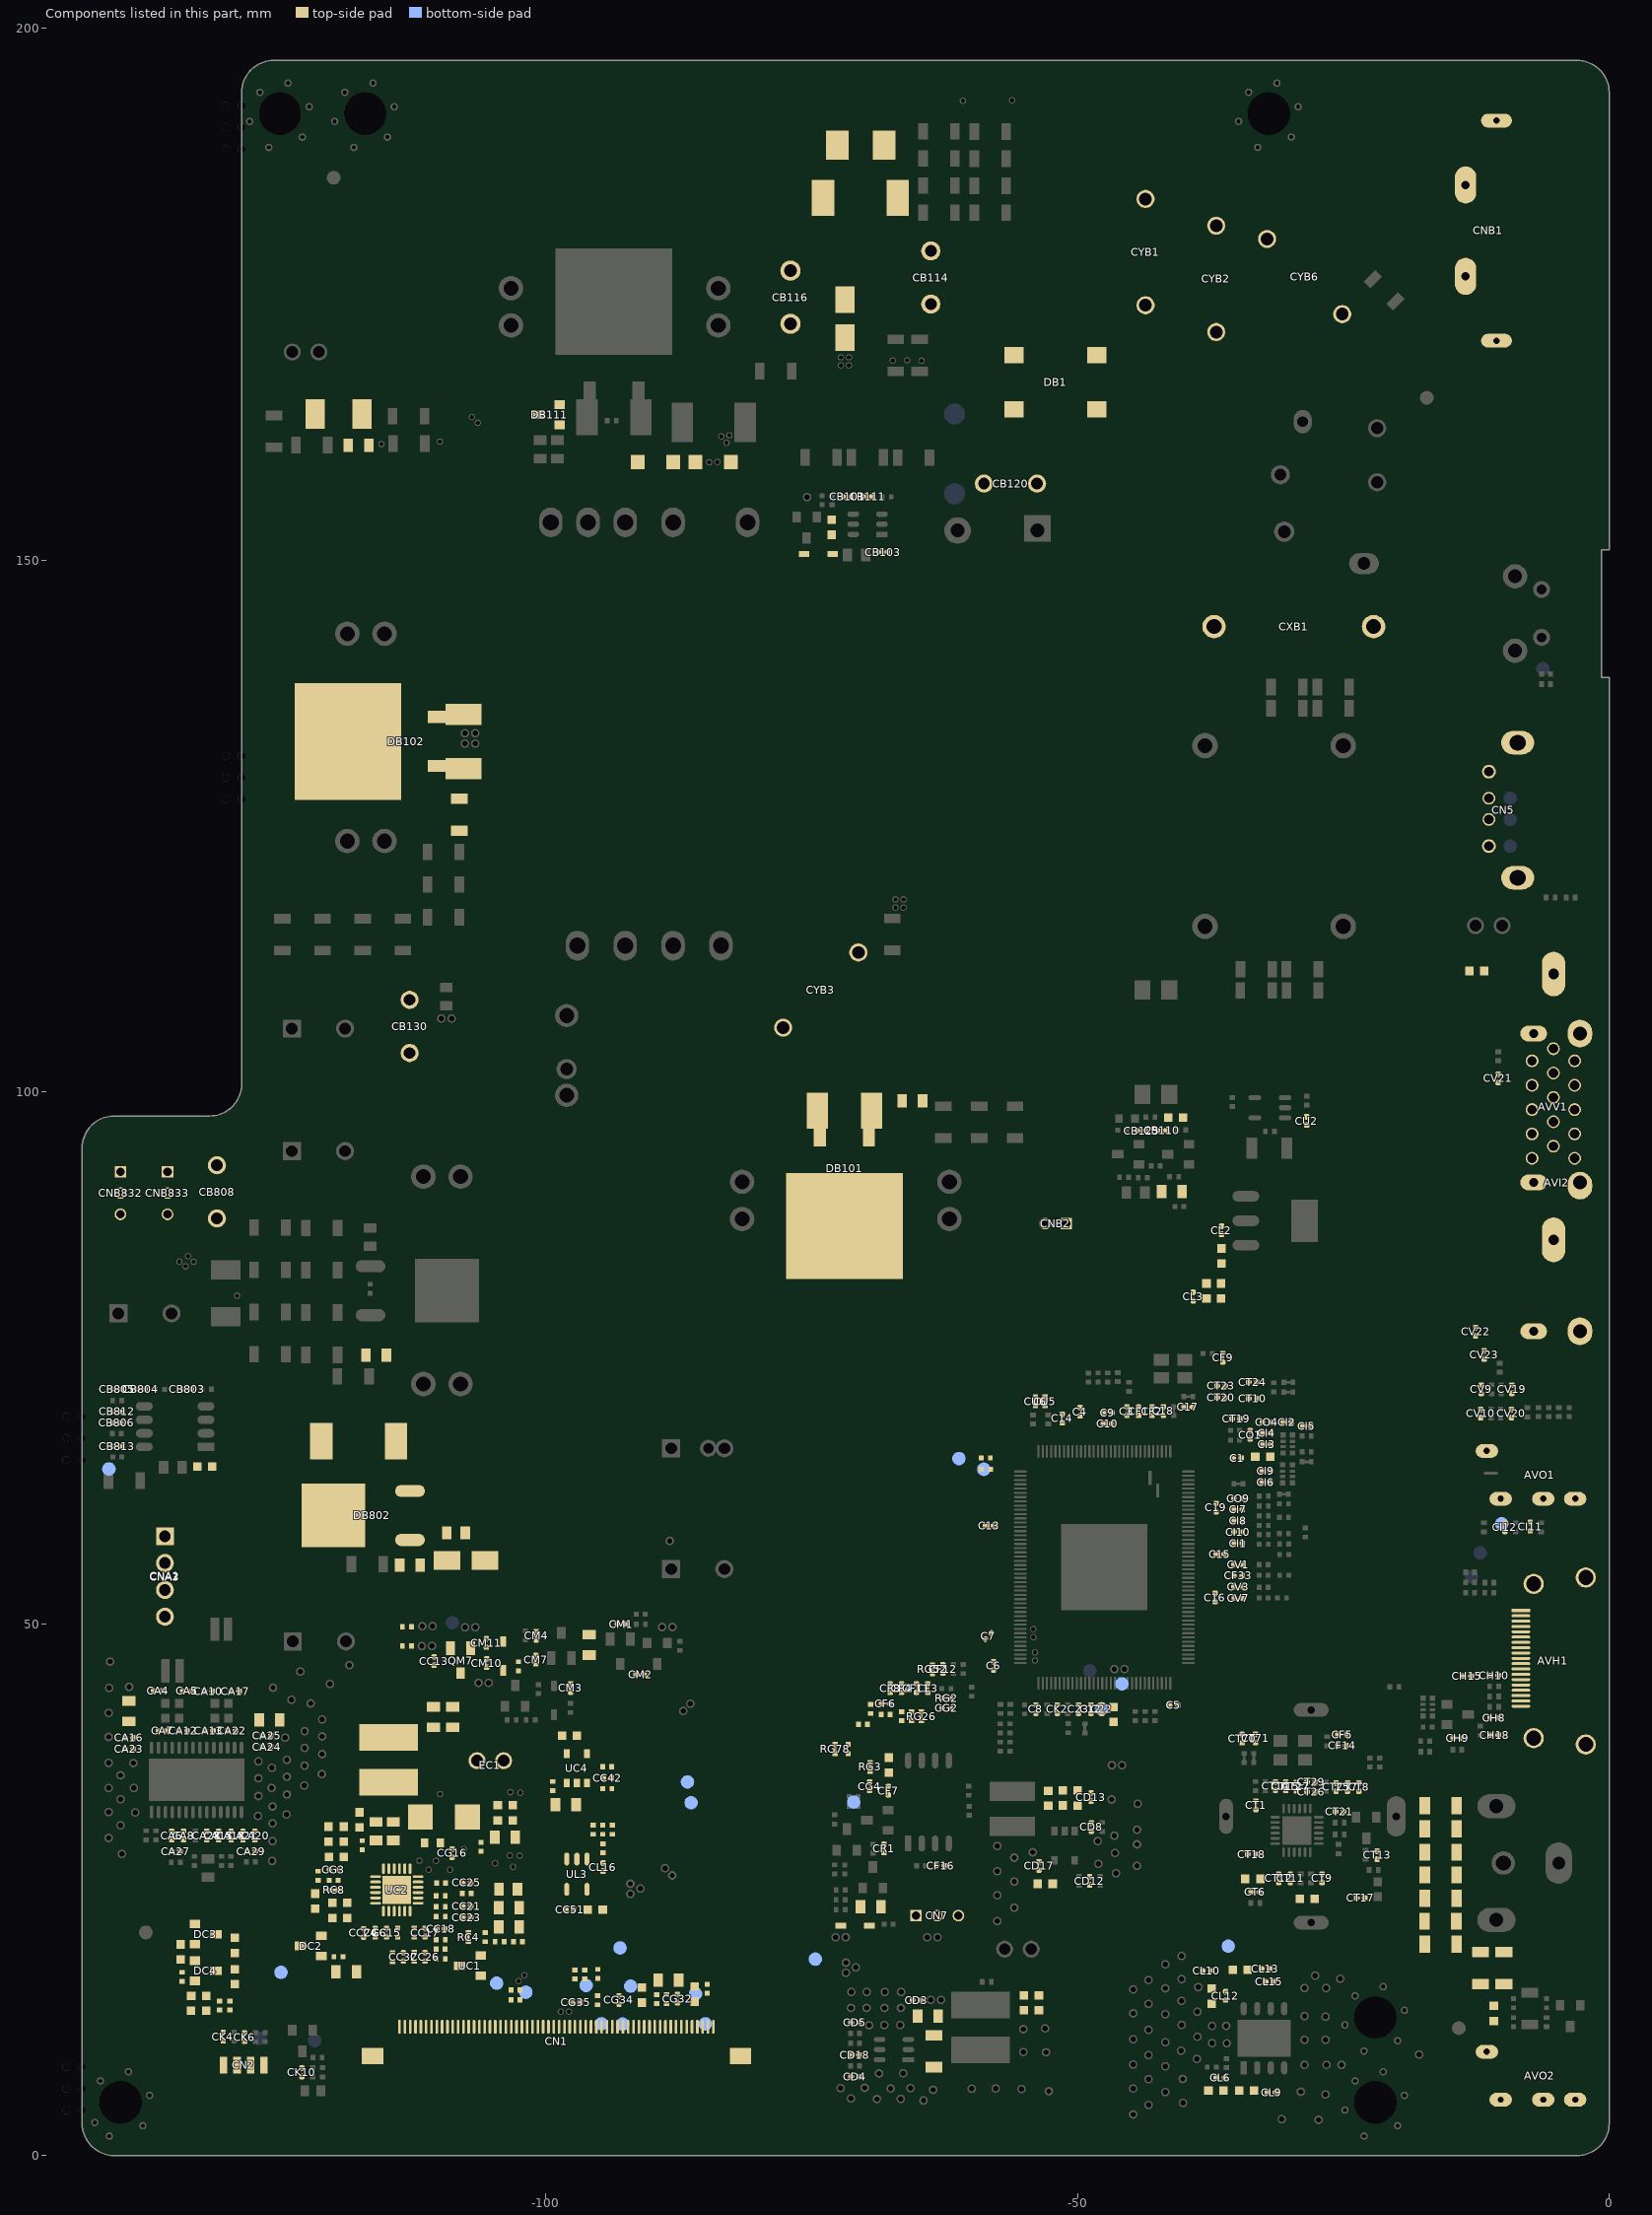
[diagram p0: the components of this part, seen from the top]
# Altium PCB MISC86383-9.PcbDoc (part 2 of 18)
Units mm, origin at the board's own origin, x right, y up, seen from the top; angles counter-clockwise.
Board outline 143.6 x 197 mm, 2 copper layers (TopLayer, BottomLayer), stack 1.571 mm thick; 743 components, 401 nets, 2996 pads, 1077 vias.
Unrouted connection lines stored in the file: 4.

## Classes and differential pairs (continued)
component class TV#08_TCON: AVDD CC1 CC2 CC4 CC5 CC7 CC8 CC9 CC10 CC11 CC12 CC13 CC15 CC17 CC18 CC19 CC20 CC21 CC23 CC24 CC25 CC26 CC27 CC29 CC30 CC31 CC32 CC33 CC34 CC38 CC42 CC43 CC50 CC51 CG3 CG4 CG6 CG14 CG16 CG22 CG28 CG31 CG32 CG33 CG34 CG35 CL16 CM10 CM11 CN1 CPV CPV2 DC1 DC2 DC3 DC4 DM3 DVDD EC1 GREF LC1 OE1 POL QM7 RC1 RC2 RC3 RC4 RC8 RC10 RC12 RC13 RC14 RC15 RC18 RC19 RC20 RC23 RC24 RC27 RC31 RC32 RC33 RC35 RC36 RG2 RG3 RG5 RG6 RG7 RG8 RG9 RG12 RG13 RG14 RG15 RG16 RG21 RG22 RG25 RG26 RG39 RG40 RG41 RG42 RG43 RG44 RG46 RG48 RG49 RG52 RG58 RG59 RG60 RG61 RG62 RG63 RG78 RG82 RGV1 RL3 RL7 RL50 RL51 RM12 STV TP TVCOM UC1 UC2 UC4 UL3 VMID/SCL VMID/SDA VOFF VON XAO
component class TV#09_LevelShif_DS8926B: RG82 STV
component class TV#10_FFC_LRbord: CNL2 CNL3
component class PS#01_XXXXXXXXXXXXXXX: "Conformal Coating" CYB5 EB107 EB801+ EB801- EVA3 EVA4 EVA5 EVA6 GL7 ML1 RB111 RB113 ZDB2
net class HOT: 12V-OVP BRO D_QB101 L L-1 L-2 L-N N N-1 N-2 N-3 NetBB101_2 NetCB101_1 NetCB103_1 NetCB113_1 NetCB113_2 NetCB114_1 NetCB114_2 NetCB116_1 NetCB116_2 NetCYB3_1 NetDB104_K NetDB106_K NetDB109_A NetDB109_K NetDB111_1 NetDB111_2 NetDB112_K NetRB101_2 NetRB106_1 NetRB141_1 NetRB143_1 NetRB144_1 NetRB150_1 SGND VBRIDGE VCC
net class POWER: 12V 12V-OVP BRO D_QB101 D_QB801 GND GND1 L L-1 L-2 L-N LED+ LED_CS LED_FB LED_GATE LED_OVP N N-1 N-2 N-3 NetBB101_2 NetBB801_2 NetBB803_1 NetCB101_1 NetCB103_1 NetCB109_1 NetCB109_2 NetCB113_1 NetCB113_2 NetCB114_1 NetCB114_2 NetCB115_1 NetCB116_1 NetCB116_2 NetCB117_1 NetCB117_2 NetCB118_1 NetCB118_2 NetCB125_1 NetCB125_2 NetCB801_2 NetCB803_1 NetCB804_1 NetCB805_2 NetCB809_1 NetCB810_2 NetCB812_2 NetCB813_2 NetCNB1_3 NetCNB1_4 NetCYB3_1 NetDB104_K NetDB106_K NetDB109_A NetDB109_K NetDB111_1 NetDB111_2 NetDB112_K NetQB105_C NetQB801_G NetRB101_2 NetRB106_1 NetRB141_1 NetRB143_1 NetRB144_1 NetRB150_1 PS_ON PWM_REF SGND STY VBL VBRIDGE VCC

## Components (designator, comment, footprint, x,y, rotation, side; value= is the part's Value field where it differs from the comment)
1.15V_STB "TEST" TP -45.822,44.348 r90 bottom
3V3_STB "TEST" TP -47.752,42.012 r180 bottom
3V3_TUNER "TEST" TP -35.82,19.686 r90 bottom
5V_STB "TEST" TP -74.651,18.466 r90 bottom
AI_V "AI_GRIPPER_V" AI_GRIPPER_V 483.311,-17.234 r270 top
AVDD "TEST" TP -101.879,15.354 r180 bottom
AVH1 "HDMI jack,HDMI Jack,H,Block up,SMD,51U019S-313HFN-E-R-F,FREEPORT" HDMI-HS-11 -0.6,46.5 r90 top locked
AVI2 "RCA jack,RCA Jack,AV3,H,Red、White、Yellow,CH5.5,D14,Seal,DIP,AV3-8.4-15C red/white/yellow,JSL" AV3-H14-15 0,91.5 r90 top locked
AVO1 "Earphone jack,Earphone Jack,H,Φ3.6,CH5.5,Black,Seal,DIP,PJ-320B-Φ5.5,JSL" PHONE-HD-43 0,64 r90 top locked
AVO2 "NC/Earphone jack,Earphone Jack,H,Φ3.6,CH5.5,Black,Seal,DIP,PJ-320B-Φ5.5,JSL" PHONE-HD-43 0,7.5 r90 top locked
AVV1 "NC/WLHD-051A" DB15-HF-1 0,98.6 r90 top locked
BB101 "Ferrite bead,BEAD,50ohm,3.0×4.0mm,9A,SMD,TP,BPH403025W4-470T,TAI-TECH" L(4*3*2.55)-S -71.882,172.733 r270 top
BB801 "Ferrite bead,BEAD,80ohm,0805,4000mA,SMD,TP,UPZ2012D800-4R0TF,Sunlord" R0805 -108.445,58.534 r180 top
BB802 "NC/Ferrite bead,BEAD,50ohm,3.0×4.0mm,9A,SMD,TP,BPH403025W4-470T,TAI-TECH" L(4*3*2.55)-S -107.505,55.956 r180 top
C1 "1uF-0402-X5R-±20%-6.3V" C0402 -34.985,65.586 r180 top
C2 "NC/10uF-0603-X5R-±20%-6.3V" C0603 -32.571,65.699 r0 top
C3 "1uF-0402-X5R-±20%-6.3V" C0402 -45.337,69.994 r270 top
C4 "1uF-0402-X5R-±20%-6.3V" C0402 -49.757,69.931 r270 top
C5 "1uF-0402-X5R-±20%-6.3V" C0402 -40.956,42.333 r180 top
C6 "Ceramic capacitor,CAP MC,16V,0.1uF,±10%,X7R,0402,SMD,TP" C0402 -57.891,46.047 r90 top
C7 "Ceramic capacitor,CAP MC,16V,0.1uF,±10%,X7R,0402,SMD,TP" C0402 -58.38,48.848 r45 top
C8 "Ceramic capacitor,CAP MC,16V,0.1uF,±10%,X7R,0402,SMD,TP" C0402 -53.91,41.978 r90 top
C9 "1uF-0402-X5R-±20%-6.3V" C0402 -47.159,69.844 r0 top
C10 "1uF-0402-X5R-±20%-6.3V" C0402 -47.165,68.815 r0 top
C11 "10uF-0603-X5R-±20%-6.3V" C0603 -46.607,41.47 r90 top
C12 "1uF-0402-X5R-±20%-6.3V" C0402 -48.728,41.978 r90 top
C13 "Ceramic capacitor,CAP MC,16V,0.1uF,±10%,X7R,0402,SMD,TP" C0402 -58.278,59.212 r0 top
C14 "Ceramic capacitor,CAP MC,16V,0.1uF,±10%,X7R,0402,SMD,TP" C0402 -51.435,69.31 r270 top
C15 "Ceramic capacitor,CAP MC,16V,0.1uF,±10%,X7R,0402,SMD,TP" C0402 -36.576,56.54 r180 top
C16 "Ceramic capacitor,CAP MC,16V,0.1uF,±10%,X7R,0402,SMD,TP" C0402 -37.059,52.476 r270 top
C17 "Ceramic capacitor,CAP MC,16V,0.1uF,±10%,X7R,0402,SMD,TP" C0402 -39.586,70.371 r0 top
C18 "Ceramic capacitor,CAP MC,16V,0.1uF,±10%,X7R,0402,SMD,TP" C0402 -41.912,70.002 r270 top
C19 "Ceramic capacitor,CAP MC,16V,0.1uF,±10%,X7R,0402,SMD,TP" C0402 -36.944,60.935 r90 top
C22 "NC/1uF-0402-X5R-±20%-6.3V" C0402 -47.725,41.978 r90 top
C23 "Ceramic capacitor,CAP MC,16V,0.1uF,±10%,X7R,0402,SMD,TP" C0402 -49.909,41.978 r90 top
CA4 "2200pF-0402-X7R-±10%-50V" C0402 -136.495,43.698 r180 top
CA5 "2200pF-0402-X7R-±10%-50V" C0402 -133.739,43.673 r0 top
CA6 "0.22uF-0402-X5R-±10%-16V" C0402 -135.182,30.084 r270 top
CA7 "0.22uF-0402-X5R-±10%-16V" C0402 -136.045,39.939 r0 top
CA8 "0.22uF-0402-X5R-±10%-16V" C0402 -134.064,30.084 r270 top
CA10 "2200pF-0402-X7R-±10%-50V" C0402 -131.732,43.66 r180 top
CA12 "0.22uF-0402-X5R-±10%-16V" C0402 -134.115,39.939 r180 top
CA13 "0.22uF-0402-X5R-±10%-16V" C0402 -131.677,39.939 r0 top
CA15 "Ceramic capacitor,CAP MC,16V,0.1uF,±10%,X7R,0402,SMD,TP" C0402 -130.762,30.084 r270 top
CA16 "NC/1000pF-0402-X7R-±10%-50V" C0402 -139.191,39.278 r0 top
CA17 "2200pF-0402-X7R-±10%-50V" C0402 -129.205,43.66 r180 top
CA18 "NC/1uF-0402-X5R-±20%-16V" C0402 -129.594,30.084 r270 top
CA20 "0.22uF-0402-X5R-±10%-16V" C0402 -127.359,30.084 r270 top
CA21 "0.22uF-0402-X5R-±10%-16V" C0402 -128.476,30.084 r270 top
CA22 "0.22uF-0402-X5R-±10%-16V" C0402 -129.543,39.939 r180 top
CA23 "NC/0.1uF-0402-X5R-±20%-16V" C0402 -139.191,38.212 r0 top
CA24 "Ceramic capacitor,CAP MC,16V,0.1uF,±10%,X7R,0402,SMD,TP" C0402 -126.233,38.427 r180 top
CA25 "NC/1000pF-0402-X7R-±10%-50V" C0402 -126.233,39.494 r180 top
CA27 "3300pF-0402-X7R-±10%-50V" C0402 -134.782,28.598 r0 top
CA28 "1uF-0402-X5R-±20%-16V" C0402 -131.88,30.084 r90 top
CA29 "3300pF-0402-X7R-±10%-50V" C0402 -127.71,28.604 r180 top
CA31 "10uF-0805-X5R-±20%-16V" C0805 -139.212,41.78 r270 top
CA32 "NC/10uF-0805-X5R-±20%-16V" C0805 -125.979,40.955 r180 top
CA36 "NC/10uF-0805-X5R-±20%-16V" C0805 -69.448,23.398 r0 top
CAUTION "CAUTION" CAUTION -173.126,207.416 r180 bottom
CB101 "100pF-0402-NPO-±5%-50V" C0402 -71.641,155.994 r0 top
CB102 "0.1uF-0603-X7R-±10%-50V" C0603 -73.114,153.111 r90 top
CB103 "Ceramic capacitor,CAP MC,50V,1000pF,±10%,X7R,0402,SMD,TP" C0402 -68.288,150.774 r180 top
CB109 "Ceramic capacitor,CAP MC,25V,0.22uF,±10%,X7R,0603,SMD,TP" C0603 -40.767,97.612 r0 top
CB110 "NC/1000pF-0402-X7R-±10%-50V" C0402 -42.062,96.393 r0 top
CB111 "NC/Ceramic capacitor,CAP MC,50V,100pF,±5%,NPO,0402,SMD,TP" C0402 -69.736,155.994 r180 top
CB113 "NC/220PF-0805-NPO-±10%-200V" C0805 -117.615,160.807 r180 top
CB114 "Film capacitor,CAP PE,400V,4700pF,±5%,P,5.0mm,PC,DIP,TP,Fara" CAP8*2.5-V-5 -63.792,176.593 r90 top
CB115 "0.1uF-0805-X7R-±10%-50V" C0805 -41.123,90.627 r180 top
CB116 "Ceramic capacitor,CAP CD,2KV,68pF,±5%,SL,IK,5.0mm,DIP,TP,Walsin" CAP6.5*5-V-5-1 -76.987,174.739 r90 top
CB117 "1000pF-0805-NPO-±10%-200V" C0805 -65.532,99.187 r0 top
CB118 "Ceramic capacitor,CAP MC,1KV,1000pF,±5%,NPO,1206,SMD,TP" C1206 -108.14,126.073 r270 top
CB120 "NC/Ceramic capacitor,CAP CD,2KV,4700pF,±20%,Y5U,IK,5.0mm,DIP,TP,Walsin" CAP10*4.5-V-5#1 -56.299,157.213 r0 top locked
CB125 "NC/Ceramic capacitor,CAP MC,50V,0.022uF,±10%,X7R,0402,SMD,TP" C0402 -43.967,96.368 r180 top
CB130 "NC/Ceramic capacitor,CAP CD,1KV,4700pF,±20%,Y5U,P,5.0mm,DIP,TP,TongHao" CAP9.8*4-V-5 -112.801,106.172 r270 top
CB801 "Ceramic capacitor,CAP MC,25V,1uF,±10%,X7R,0603,SMD,TP" C0603 -132.067,64.795 r180 top
CB803 "100pF-0402-NPO-±5%-50V" C0402 -133.737,72.074 r180 top
CB804 "4700pF-0402-X7R-±10%-50V" C0402 -138.074,72.06 r180 top
CB805 "NC/0.1uF-0402-X7R-±10%-16V" C0402 -140.31,72.047 r180 top
CB806 "Ceramic capacitor,CAP MC,50V,1000pF,±10%,X7R,0402,SMD,TP" C0402 -140.345,68.885 r180 top
CB808 "NC/Ceramic capacitor,CAP CD,1KV,4700pF,±20%,Y5U,K,5.0mm,DIP,TP,Walsin" CAP10*4.5-V-5#2 -130.924,90.614 r90 top
CB809 "Ceramic capacitor,CAP MC,500V,220pF,±5%,NPO,0805,SMD,TP" C0805 -115.951,75.248 r0 top
CB810 "Ceramic capacitor,CAP MC,500V,220pF,±5%,NPO,0805,SMD,TP" C0805 -112.776,55.499 r180 top
CB812 "0.033uF-0402-X7R-±10%-16V" C0402 -140.341,69.952 r0 top
CB813 "100pF-0402-NPO-±5%-50V" C0402 -140.319,66.675 r0 top
CC1 "NC/Ceramic capacitor,CAP MC,25V,10uF,±10%,X5R,0805,SMD,TP" C0805 -103.454,21.483 r180 top
CC2 "Ceramic capacitor,CAP MC,25V,10uF,±10%,X5R,0805,SMD,TP" C0805 -103.454,23.312 r180 top
CC4 "Ceramic capacitor,CAP MC,25V,1uF,±10%,X7R,0603,SMD,TP" C0603 -118.681,23.05 r90 top
CC5 "Ceramic capacitor,CAP MC,16V,2.2uF,±10%,X5R,0603,SMD,TP" C0603 -121.672,23.919 r270 top
CC7 "Ceramic capacitor,CAP MC,50V,0.1uF,±10%,X7R,0603,SMD,TP" C0603 -120.053,23.05 r270 top
CC8 "Ceramic capacitor,CAP MC,16V,10uF,±20%,X5R,0805,SMD,TP" C0805 -108.753,41.219 r90 top
CC9 "NC/0.1uF-0603-X7R-±10%-50V" C0603 -118.999,30.226 r90 top
CC10 "Ceramic capacitor,CAP MC,50V,0.1uF,±10%,X7R,0603,SMD,TP" C0603 -120.421,30.226 r90 top
CC11 "Ceramic capacitor,CAP MC,50V,0.1uF,±10%,X7R,0603,SMD,TP" C0603 -119.697,28.092 r180 top
CC12 "NC/Ceramic capacitor,CAP MC,16V,10uF,±20%,X5R,0805,SMD,TP" C0805 -110.582,41.219 r90 top
CC13 "NC/0.1uF-0402-X5R-±20%-16V" C0402 -110.503,46.495 r270 top
CC15 "1uF-0402-X5R-±20%-6.3V" C0402 -114.98,20.955 r270 top
CC17 "1uF-0402-X5R-±20%-6.3V" C0402 -111.36,20.955 r90 top
CC18 "1uF-0402-X5R-±20%-6.3V" C0402 -109.884,21.302 r180 top
CC19 "Ceramic capacitor,CAP MC,25V,10uF,±10%,X5R,0805,SMD,TP" C0805 -103.835,29.909 r0 top
CC20 "Ceramic capacitor,CAP MC,25V,1uF,±10%,X7R,0603,SMD,TP" C0603 -103.81,32.944 r0 top
CC21 "Ceramic capacitor,CAP MC,50V,1000pF,±10%,X7R,0402,SMD,TP" C0402 -107.444,23.463 r0 top
CC23 "NC/0.1uF-0402-X5R-±20%-16V" C0402 -107.444,22.396 r180 top
CC24 "Ceramic capacitor,CAP MC,16V,0.1uF,±10%,X7R,0402,SMD,TP" C0402 -117.129,20.937 r270 top
CC25 "NC/33pF-0402-NPO-±5%-50V" C0402 -107.449,25.645 r0 top
CC26 "NC/33pF-0402-NPO-±5%-50V" C0402 -111.36,18.669 r270 top
CC27 "Ceramic capacitor,CAP MC,50V,0.1uF,±10%,X7R,0603,SMD,TP" C0603 -129.235,19.761 r270 top
CC29 "10uF-0805-X5R-±20%-16V" C0805 -88.468,16.485 r0 top
CC30 "NC/10uF-0805-X5R-±20%-16V" C0805 -118.77,17.259 r0 top
CC31 "Ceramic capacitor,CAP MC,50V,0.1uF,±10%,X7R,0603,SMD,TP" C0603 -129.235,16.815 r90 top
CC32 "NC/33pF-0402-NPO-±5%-50V" C0402 -113.392,18.669 r270 top
CC33 "1uF-0603-X5R-±10%-50V" C0603 -132.639,15.011 r0 top
CC34 "Ceramic capacitor,CAP MC,50V,0.1uF,±10%,X7R,0603,SMD,TP" C0603 -132.651,13.614 r0 top
CC38 "Ceramic capacitor,CAP MC,50V,0.1uF,±10%,X7R,0603,SMD,TP" C0603 -97.777,39.484 r180 top
CC42 "Ceramic capacitor,CAP MC,16V,0.1uF,±10%,X7R,0402,SMD,TP" C0402 -94.208,35.496 r0 top
CC43 "10uF-0805-X5R-±20%-16V" C0805 -98.12,32.982 r180 top
CC50 "NC/10uF-0603-X5R-±20%-6.3V" C0603 -95.352,23.114 r0 top
CC51 "1uF-0402-X5R-±20%-6.3V" C0402 -97.739,23.114 r0 top
CD1 "Ceramic capacitor,CAP MC,16V,10uF,±10%,X5R,1206,SMD,TP" C1206 -63.5,9.804 r90 top
CD2 "10uF-0805-X5R-±20%-16V" C0805 -64.059,13.106 r180 top
CD3 "NC/Ceramic capacitor,CAP MC,16V,0.1uF,±10%,X7R,0402,SMD,TP" C0402 -65.126,14.605 r0 top
CD4 "Ceramic capacitor,CAP MC,16V,0.1uF,±10%,X7R,0402,SMD,TP" C0402 -70.917,7.417 r0 top
CD5 "NC/Ceramic capacitor,CAP MC,50V,470pF,±5%,NPO,0402,SMD,TP" C0402 -70.918,12.49 r180 top
CD7 "Ceramic capacitor,CAP MC,10V,10uF,±20%,X5R,0603,SMD,TP" C0603 -54.334,15.056 r180 top
CD8 "Ceramic capacitor,CAP MC,16V,0.1uF,±10%,X7R,0402,SMD,TP" C0402 -48.701,30.889 r270 top
CD9 "NC/Ceramic capacitor,CAP MC,10V,10uF,±20%,X5R,0603,SMD,TP" C0603 -54.329,13.672 r180 top
CD10 "NC/10uF-0603-X5R-±20%-6.3V" C0603 -49.974,33.617 r90 top
CD12 "NC/NC/3300pF-0402-X7R-±10%-50V" C0402 -48.854,25.82 r270 top
CD13 "NC/0.1uF-0402-X5R-±20%-16V" C0402 -48.717,33.693 r90 top
CD14 "10uF-0603-X5R-±20%-6.3V" C0603 -52.751,33.594 r90 top
CD15 "10uF-0603-X5R-±20%-6.3V" C0603 -51.372,33.624 r90 top
CD16 "10uF-0603-X5R-±20%-6.3V" C0603 -53.035,25.552 r180 top
CD17 "NC/0.1uF-0402-X5R-±20%-16V" C0402 -53.619,27.229 r270 top
CD18 "NC/0.1uF-0402-X5R-±20%-16V" C0402 -70.92,9.451 r0 top
CF1 "Ceramic capacitor,CAP MC,50V,18pF,±5%,NPO,0402,SMD,TP" C0402 -44.249,69.978 r270 top
CF2 "Ceramic capacitor,CAP MC,50V,18pF,±5%,NPO,0402,SMD,TP" C0402 -42.979,69.989 r270 top
CF3 "NC/1000pF-0402-X7R-±10%-50V" C0402 -64.069,43.946 r270 top
CF4 "NC/1000pF-0402-X7R-±10%-50V" C0402 -66.548,43.942 r270 top
CF5 "NC/0ohm-0402-PCB" R0402SC -25.11,39.563 r180 top
CF6 "NC/1000pF-0402-X7R-±10%-50V" C0402 -68.047,42.469 r180 top
CF7 "Ceramic capacitor,CAP MC,16V,0.1uF,±10%,X7R,0402,SMD,TP" C0402 -67.783,34.296 r270 top
CF8 "NC/1000pF-0402-X7R-±10%-50V" C0402 -67.615,43.942 r270 top
CF9 "NC/30pF-0402-NPO-±5%-50V" C0402 -36.332,75.01 r90 top
CF10 "NC/10uF-0603-X5R-±20%-6.3V" C0603 -67.755,36.704 r270 top
CF11 "NC/1000pF-0402-X7R-±10%-50V" C0402 -65.151,43.942 r270 top
CF12 "NC/1000pF-0402-X7R-±10%-50V" C0402 -62.649,45.745 r270 top
CF14 "NC/4.7pF-0402-NPO-±5%-50V" C0402 -25.11,38.547 r180 top
CF16 "NC/0.1uF-0402-X5R-±20%-16V" C0402 -62.884,27.254 r0 top
CF33 "NC/0.047uF-0402-X7R-±10%-16V" C0402 -34.891,54.523 r0 top
CG2 "NC/Ceramic capacitor,CAP MC,16V,0.1uF,±10%,X7R,0402,SMD,TP" C0402 -62.332,42.05 r180 top
CG3 "Ceramic capacitor,CAP MC,16V,0.1uF,±10%,X7R,0402,SMD,TP" C0402 -119.958,26.878 r0 top
CG4 "NC/Ceramic capacitor,CAP MC,16V,0.1uF,±10%,X7R,0402,SMD,TP" C0402 -69.545,34.722 r270 top
CG6 "NC/1uF-0402-X5R-±20%-6.3V" C0402 -116.046,20.955 r270 top
CG14 "NC/0.1uF-0603-X7R-±10%-50V" C0603 -117.5,31.559 r90 top
CG16 "Ceramic capacitor,CAP MC,50V,33pF,±5%,NPO,0402,SMD,TP" C0402 -108.814,28.435 r90 top
CG22 "NC/1uF-0603-X5R-±10%-50V" C0603 -103.81,31.521 r0 top
CG28 "1uF-0603-X5R-±10%-50V" C0603 -134.353,19.139 r90 top
CG31 "10uF-0603-X5R-±20%-6.3V" C0603 -85.992,15.176 r90 top
CG32 "NC/0.1uF-0402-X5R-±20%-16V" C0402 -87.617,14.745 r270 top
CG33 "NC/0.1uF-0603-X7R-±10%-50V" C0603 -90.957,15.088 r270 top
CG34 "NC/0.1uF-0402-X5R-±20%-16V" C0402 -93.116,14.618 r270 top
CG35 "NC/Ceramic capacitor,CAP MC,25V,0.1uF,±20%,X5R,0402,SMD,TP" C0402 -97.168,14.402 r0 top
CH8 "NC/0.1uF-0402-X5R-±20%-16V" C0402 -10.821,41.166 r0 top
CH9 "NC/0.1uF-0402-X5R-±20%-16V" C0402 -14.275,39.261 r180 top
CH10 "NC/30pF-0402-NPO-±5%-50V" C0402 -10.82,45.148 r0 top
CH15 "NC/1uF-0402-X5R-±20%-16V" C0402 -13.373,45.072 r180 top
CH18 "NC/0.1uF-0402-X7R-±10%-16V" C0402 -10.796,39.54 r180 top
CI1 "NC/0.047uF-0402-X7R-±10%-16V" C0402 -34.882,57.571 r0 top
CI2 "NC/4700pF-0402-X7R-±10%-16V" C0402 -30.281,68.963 r180 top
CI3 "NC/0.1uF-0402-X5R-±20%-16V" C0402 -32.203,66.874 r0 top
CI4 "NC/0.1uF-0402-X5R-±20%-16V" C0402 -32.203,67.935 r0 top
CI5 "NC/4700pF-0402-X7R-±10%-16V" C0402 -28.447,68.595 r180 top
CI6 "Ceramic capacitor,CAP MC,16V,0.1uF,±10%,X7R,0402,SMD,TP" C0402 -32.267,63.29 r0 top
CI7 "0.047uF-0402-X7R-±10%-16V" C0402 -34.882,60.734 r0 top
CI8 "0.047uF-0402-X7R-±10%-16V" C0402 -34.882,59.705 r0 top
CI9 "Ceramic capacitor,CAP MC,16V,0.1uF,±10%,X7R,0402,SMD,TP" C0402 -32.267,64.357 r0 top
CI10 "0.047uF-0402-X7R-±10%-16V" C0402 -34.882,58.638 r0 top
CI11 "NC/1000pF-0402-X7R-±10%-50V" C0402 -7.417,59.131 r270 top
CI12 "NC/4700pF-0402-X7R-±10%-50V" C0402 -9.804,59.08 r270 top
CK2 "Ceramic capacitor,CAP MC,50V,0.01uF,±10%,X7R,0402,SMD,TP" C0402 -51.903,41.978 r270 top
CK4 "Ceramic capacitor,CAP MC,16V,0.1uF,±10%,X7R,0402,SMD,TP" C0402 -130.333,11.174 r90 top
CK6 "NC/10pF-0402-NPO-±5%-50V" C0402 -128.321,11.125 r90 top
CK10 "NC/0.1uF-0402-X5R-±20%-16V" C0402 -122.936,7.823 r270 top
CL1 "NC/10uF-0603-X5R-±20%-6.3V" C0603 -36.449,84.582 r90 top
CL2 "Ceramic capacitor,CAP MC,16V,0.1uF,±10%,X7R,0402,SMD,TP" C0402 -36.449,86.991 r270 top
CL3 "Ceramic capacitor,CAP MC,6.3V,1uF,±20%,X5R,0402,SMD,TP" C0402 -39.116,80.772 r270 top
CL4 "NC/10uF-0603-X5R-±20%-6.3V" C0603 -36.5,81.297 r270 top
CL5 "NC/10uF-0603-X5R-±20%-6.3V" C0603 -37.871,81.297 r270 top
CL6 "Ceramic capacitor,CAP MC,16V,0.1uF,±10%,X7R,0402,SMD,TP" C0402 -36.551,7.315 r0 top
CL7 "NC/10uF-0603-X5R-±20%-6.3V" C0603 -36.982,6.096 r0 top
CL8 "NC/10uF-0603-X5R-±20%-6.3V" C0603 -34.087,6.096 r0 top
CL9 "Ceramic capacitor,CAP MC,16V,0.1uF,±10%,X7R,0402,SMD,TP" C0402 -31.75,5.944 r180 top
CL10 "NC/Ceramic capacitor,CAP MC,16V,0.1uF,±10%,X7R,0402,SMD,TP" C0402 -37.846,17.374 r0 top
CL11 "NC/10uF-0603-X5R-±20%-6.3V" C0603 -37.389,14.986 r270 top
CL12 "Ceramic capacitor,CAP MC,6.3V,1uF,±20%,X5R,0402,SMD,TP" C0402 -36.068,15.011 r90 top
CL13 "NC/Ceramic capacitor,CAP MC,16V,0.1uF,±10%,X7R,0402,SMD,TP" C0402 -32.309,17.577 r0 top
CL14 "NC/10uF-0603-X5R-±20%-6.3V" C0603 -34.696,17.475 r180 top
CL15 "Ceramic capacitor,CAP MC,6.3V,1uF,±20%,X5R,0402,SMD,TP" C0402 -31.953,16.358 r0 top
CL16 "Ceramic capacitor,CAP MC,16V,0.1uF,±10%,X7R,0402,SMD,TP" C0402 -94.615,27.114 r270 top
CM1 "0.22uF-0402-X5R-±10%-16V" C0402 -92.9,49.974 r0 top
CM2 "Ceramic capacitor,CAP MC,16V,0.1uF,±10%,X7R,0402,SMD,TP" C0402 -91.122,45.212 r0 top
CM3 "NC/Ceramic capacitor,CAP MC,16V,0.1uF,±10%,X7R,0402,SMD,TP" C0402 -97.665,43.963 r270 top
CM4 "Ceramic capacitor,CAP MC,16V,0.1uF,±10%,X7R,0402,SMD,TP" C0402 -100.901,48.87 r270 top
CM5 "NC/10uF-0805-X5R-±20%-16V" C0805 -95.936,48.019 r270 top
CM7 "0.022uF-0402-X7R-±10%-16V" C0402 -100.94,46.622 r90 top
CM10 "NC/0.022uF-0402-X7R-±10%-50V" C0402 -105.55,46.304 r90 top
CM11 "Ceramic capacitor,CAP MC,16V,0.22uF,±20%,X5R,0402,SMD,TP" C0402 -105.588,48.197 r90 top
CN1 "FFC connector,FFC connector,60Pin,D0.5,Bottom,lock,SMD,0.5-22-60PBX-P,XFE" FFC60H/0.5S-11 -99,10.728 r0 top locked
CN2 "IR receiver transistor,IR Receriver,2.7-5.5V,37.9KHz,SMD,SIRAB39R1,SL" REMOTE-HS-1 -128.4,6.23 r0 top locked
CN5 "USB jack,USB Jack,USB2.0,H,Single,Black,flange,Block up,DIP,103411481,VAST" USB-HD-30 -0.5,126.5 r90 top locked
CN7 "Connector socket,connect jack,3Pin,D2.0,D,SNAP,L=2.8mm,DIP,CNJST" SIP3/2.0D-3 -63.195,22.555 r0 top
CNA1 "NC/4PIN-2.54-D-H-G" SIP4/2.54D-1 -135.814,54.475 r270 top
CNA2 "Connector socket,connect jack,4PIN,D2.50,L,SNAP,STEP,Fool-proofing,Nature,L=3.0mm,DIP,AMA" SIP4H/2.5D-7 -135.994,54.445 r270 top
CNA3 "NC/Connector socket,connect jack,4Pin,D2.5,D,SNAP,Nature,L=2.8mm,DIP,W2411-04SVA-S03-E,XYDT" SIP4/2.5D-2 -135.814,54.415 r270 top
CNB1 "Red-phosphorus-free connector socket,connect jack(HP),2Pin,D8.6,L,SNAP,Fool-proofing,Black,L=4.0mm,DIP,YQ" CON2-H8.6-1 -14,181 r90 top locked
CNB2 "Connector socket,connect jack,2Pin,D2.0,D,Beige,L=2.8mm,DIP,W2011-02SVA-SN8-ENSY,XYDT" SIP2/2.0D-1 -52.054,87.63 r180 top
CNB832 "NC/Connector socket,connect jack,3Pin,D2.0,D,SNAP,L=2.8mm,DIP,CNJST" SIP3/2.0D-CP -140,90.5 r270 top locked
CNB833 "Connector socket,connect jack,3Pin,D2.0,L,SNAP,STEP,Fool-proofing,nature,L=2.8mm,DIP,CNJST" SIP3H/2.0D-3 -135.57,90.5 r270 top locked
CO1 "0.47uF-0402-X5R-±10%-6.3V" C0402 -33.752,67.77 r270 top
CO4 "0.47uF-0402-X5R-±10%-6.3V" C0402 -32.208,68.951 r180 top
CO9 "Ceramic capacitor,CAP MC,50V,100pF,±5%,NPO,0402,SMD,TP" C0402 -34.882,61.788 r180 top
CO77 "NC/10uF-0603-X5R-±20%-6.3V" C0603 -10.846,13.365 r270 top
COLD "COLD" COLD -70.612,61.468 r0 top
CPV "TEST" TP -71.044,33.236 r180 bottom
CPV2 "TEST" TP -85.001,12.383 r180 bottom
CQC "CQC" CQC -22.197,67.314 r0 top
CR1 "NC/1uF-0402-X5R-±20%-16V" C0402 -68.191,28.866 r270 top
CT1 "Ceramic capacitor,CAP MC,16V,0.1uF,±10%,X7R,0402,SMD,TP" C0402 -33.225,32.933 r90 top
CT2 "10uF-0603-X5R-±20%-6.3V" C0603 -28.386,24.132 r180 top
CT5 "NC/10uF-0603-X5R-±20%-6.3V" C0603 -33.517,26.012 r0 top
CT6 "Ceramic capacitor,CAP MC,16V,0.1uF,±10%,X7R,0402,SMD,TP" C0402 -33.289,24.767 r180 top
CT7 "Ceramic capacitor,CAP MC,50V,22pF,±5%,NPO,0402,SMD,TP" C0402 -24.597,34.648 r270 top
CT8 "Ceramic capacitor,CAP MC,50V,22pF,±5%,NPO,0402,SMD,TP" C0402 -23.53,34.648 r270 top
CT9 "Ceramic capacitor,CAP MC,16V,0.1uF,±10%,X7R,0402,SMD,TP" C0402 -26.997,26.062 r270 top
CT10 "30pF-0402-NPO-±5%-50V" C0402 -33.521,71.184 r0 top
CT11 "0.022uF-0402-X7R-±10%-16V" C0402 -29.987,26.062 r90 top
CT12 "0.022uF-0402-X7R-±10%-16V" C0402 -31.067,26.062 r270 top
CT13 "NC/1.2pF-0402-NPO-±0.25pf-50V" C0402 -21.831,28.24 r90 top
CT14 "NC/8pF-0402-NPO-±5%-50V" C0402 -31.379,34.736 r90 top
CT15 "NC/8pF-0402-NPO-±5%-50V" C0402 -30.414,34.711 r270 top
CT17 "NC/180pF-0402-NPO-±5%-50V" C0402 -23.374,24.216 r180 top
CT18 "Ceramic capacitor,CAP MC,16V,0.1uF,±10%,X7R,0402,SMD,TP" C0402 -33.614,28.323 r0 top
CT19 "0.022uF-0402-X7R-±10%-16V" C0402 -35.085,69.27 r180 top
CT20 "Ceramic capacitor,CAP MC,16V,0.1uF,±10%,X7R,0402,SMD,TP" C0402 -36.487,71.26 r180 top
CT21 "0.047uF-0402-X7R-±10%-16V" C0402 -25.372,32.348 r0 top
CT23 "Ceramic capacitor,CAP MC,16V,0.1uF,±10%,X7R,0402,SMD,TP" C0402 -36.487,72.371 r180 top
CT24 "30pF-0402-NPO-±5%-50V" C0402 -33.521,72.721 r180 top
CT25 "Ceramic capacitor,CAP MC,16V,0.1uF,±10%,X7R,0402,SMD,TP" C0402 -25.677,34.648 r90 top
CT26 "330pF-0402-NPO-±5%-50V" C0402 -28.026,34.203 r0 top
CT27 "Ceramic capacitor,CAP MC,16V,0.1uF,±10%,X7R,0402,SMD,TP" C0402 -29.436,34.698 r90 top
CT29 "6800pF-0402-X7R-±10%-50V" C0402 -28.026,35.13 r0 top
CT40 "Ceramic capacitor,CAP MC,1KV,470pF,±5%,NPO,1206,SMD,TP" C1206 -15.849,24.193 r180 top
CT41 "Ceramic capacitor,CAP MC,1KV,4700pF,±10%,X7R,1206,SMD,TP" C1206 -15.85,26.378 r0 top
CT42 "Ceramic capacitor,CAP MC,1KV,4700pF,±10%,X7R,1206,SMD,TP" C1206 -15.863,22.022 r0 top
CT43 "Ceramic capacitor,CAP MC,1KV,4700pF,±10%,X7R,1206,SMD,TP" C1206 -15.85,19.875 r0 top
CT44 "Ceramic capacitor,CAP MC,1KV,4700pF,±10%,X7R,1206,SMD,TP" C1206 -15.85,28.511 r0 top
CT45 "Ceramic capacitor,CAP MC,1KV,4700pF,±10%,X7R,1206,SMD,TP" C1206 -12.09,17.628 r90 top
CT46 "Ceramic capacitor,CAP MC,1KV,4700pF,±10%,X7R,1206,SMD,TP" C1206 -15.85,30.709 r0 top
CT47 "NC/Ceramic capacitor,CAP MC,1KV,4700pF,±10%,X7R,1206,SMD,TP" C1206 -9.906,17.628 r90 top
CT48 "NC/Ceramic capacitor,CAP MC,1KV,4700pF,±10%,X7R,1206,SMD,TP" C1206 -15.85,32.893 r0 top
CT70 "NC/30pF-0402-NPO-±5%-50V" C0402 -34.52,39.204 r90 top
CT71 "NC/30pF-0402-NPO-±5%-50V" C0402 -33.266,39.23 r270 top
CU1 "NC/10uF-0603-X5R-±20%-6.3V" C0603 -12.446,111.379 r180 top
CU2 "Ceramic capacitor,CAP MC,6.3V,0.47uF,±10%,X5R,0402,SMD,TP" C0402 -28.448,97.286 r90 top
CU5 "NC/0ohm-0402-PCB" R0402SC -53.035,70.907 r270 top
CU6 "NC/0ohm-0402-PCB" R0402SC -53.95,70.907 r270 top
CV1 "NC/0.047uF-0402-X7R-±10%-16V" C0402 -34.883,55.547 r0 top
CV3 "NC/0.047uF-0402-X7R-±10%-16V" C0402 -34.883,53.464 r0 top
CV7 "NC/0.047uF-0402-X7R-±10%-16V" C0402 -34.87,52.397 r0 top
CV9 "NC/33pF-0402-NPO-±5%-50V" C0402 -12.032,72.056 r270 top
CV10 "NC/33pF-0402-NPO-±5%-50V" C0402 -12.084,69.775 r270 top
CV19 "NC/33pF-0402-NPO-±5%-50V" C0402 -9.155,72.056 r90 top
CV20 "NC/33pF-0402-NPO-±5%-50V" C0402 -9.195,69.78 r90 top
CV21 "NC/33pF-0402-NPO-±5%-50V" C0402 -10.44,101.289 r270 top
CV22 "NC/33pF-0402-NPO-±5%-50V" C0402 -12.56,77.47 r270 top
CV23 "NC/33pF-0402-NPO-±5%-50V" C0402 -11.747,75.286 r270 top
CVBS_IN/OUT "TEST" TP -10.108,59.398 r90 bottom
CXB1 "X capacitor,CAP X2,MP,275VAC,0.47uF,±10%,S,15mm-Mini,PC,DIP,BM" CAP18*8.5-V-15 -29.654,143.764 r180 top
CYB1 "Y capacitor,CAP Y1,CD,470pF,400VAC,±20%,K,10mm,Y5U,DIP,TP,Walsin" CAP13*5-V-10-1 -43.599,178.981 r90 top locked
CYB2 "Y capacitor,CAP Y1,CD,470pF,400VAC,±20%,K,10mm,Y5U,DIP,TP,Walsin" CAP13*5-V-10-1 -36.957,176.466 r90 top locked
CYB3 "Y capacitor,CAP Y1,CD,470pF,400VAC,±20%,K,10mm,Y5U,DIP,TP,Walsin" CAP13*5-V-10-1 -74.143,109.588 r225 top
CYB6 "NC/Y capacitor,CAP Y1,CD,47pF,400VAC,±5%,KS,10mm,SL,DIP,BULK,Walsin" CAP13*5-V-10-1 -28.639,176.682 r135 top locked
DA1 "NC/1N4148WS" DIODE-S-12 -70.917,21.615 r180 top
DAS1 "35.0*5.4mm" DOLBY_AS2 -101.6,0.889 r0 top
DB1 "Bridge rectifier,DIO BRD,3A,800V,YBS,SMD,YBS3010A,YJ" B/YBS3010A -52.07,166.751 r90 top
DB101 "Schottky diode,DIO SBD D1,10A,150V,TO-263,SMD,HBR10150SS,JLHW" D2PAK3 -71.818,90.754 r90 top
DB102 "Schottky diode,DIO SBD D1,10A,200V,TO-263,SMD,HBR10200SS,JLHW" D2PAK3 -115.24,132.867 r0 top
DB104 "Rectifier diode,DIO SI S,1A,1000V,SMAF,SMD,M7F,YJ" DIODE-S-2 -119.494,163.766 r180 top
DB106 "NC/Rectifier diode,DIO SI S,3A,1000V,SMC,SMD,GS3M,GULF" DIODE-SMC -70.421,184.086 r180 top
DB107 "Rectifier diode,DIO FRD S,3A,1000V,SMB,SMD,GR3MBS,YJ" DIODE-SMB -70.383,189.039 r180 top
DB109 "Rectifier diode,DIO FRD S,1.2A,800V,SOD-123FL,SMD,F1K,YJ" DIODE-S-14 -89.7,159.22 r180 top
DB110 "Rectifier diode,DIO FRD S,1.2A,800V,SOD-123FL,SMD,F1K,YJ" DIODE-S-14 -84.264,159.22 r180 top
DB111 "Switching diode,DIO SW D1,215mA,85V,SOT-23,SMD,KAV70,KEXIN" SO-23 -99.708,163.69 r270 top
DB112 "Switching diode,DIO SW S,200mA,250V,SOD-323,SMD,BAV21WS,BLUE ROCKET" DIODE-S-12 -74.371,150.609 r180 top
DB801 "Schottky diode,DIO SBD S,3A,100V,SMC,SMD,SS310,YJ" DIODE-SMC -117.602,67.17 r0 top
DB802 "NC/Schottky diode,DIO SBD D1,10A,150V,TO-252,SMD,MBRD10150CT,GOOD-ARK" TO-252 -116.37,60.185 r90 top